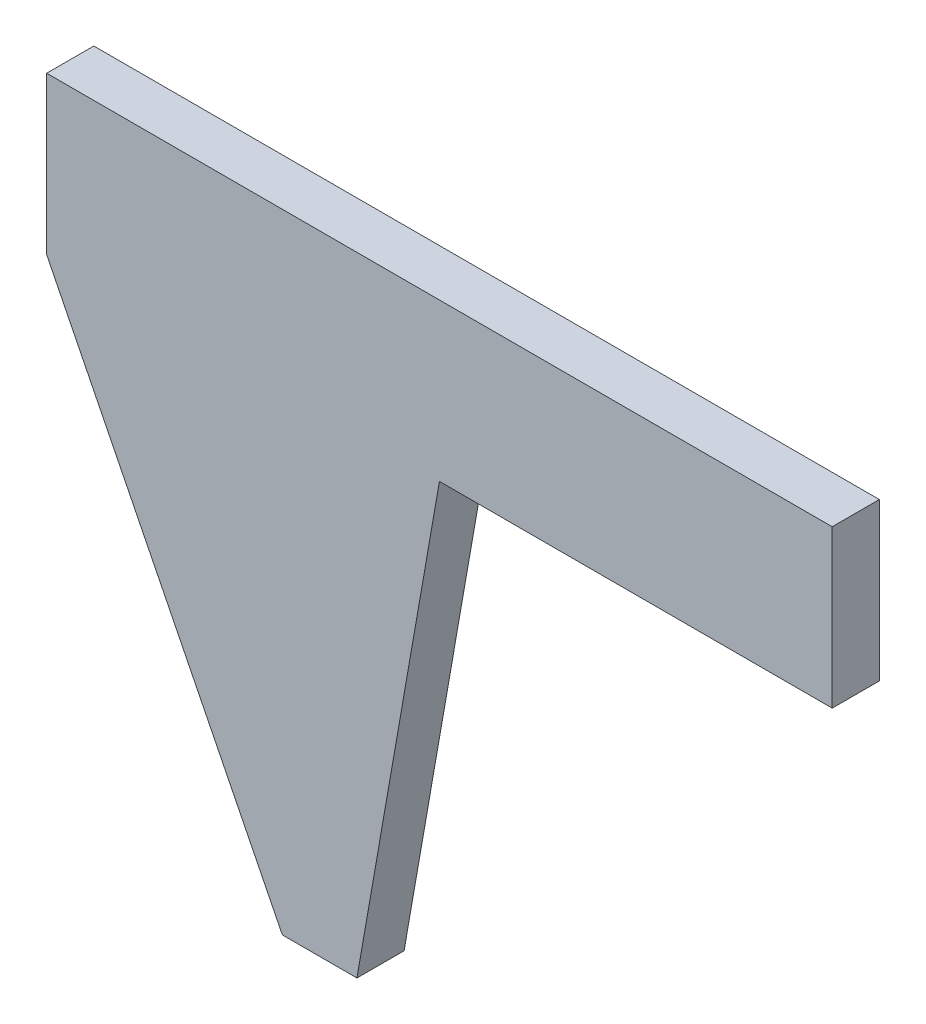
from build123d import *

# Parameters (mm, degrees)
SKETCH_1_W          = 200
SKETCH_1_H          = 160
EXTRUDE_1_DEPTH     = 12
CUT_EXTRUDE_1_DEPTH = 12


with BuildPart() as part:
    # 草图1 → 凸台-拉伸1 (new body)
    with BuildSketch(Plane.XY):
        Rectangle(SKETCH_1_W, SKETCH_1_H)
    extrude(amount=EXTRUDE_1_DEPTH)

    # 草图2 → 切除-拉伸1 (cut)
    with BuildSketch(Plane.XY.offset(12)):
        Polygon((-100, 40), (-40, -80), (-100, -80), align=None)
        Polygon((-21, -80), (0, 40), (100, 40), (100, -80), align=None)
    extrude(amount=-CUT_EXTRUDE_1_DEPTH, mode=Mode.SUBTRACT)


solid = part.part
